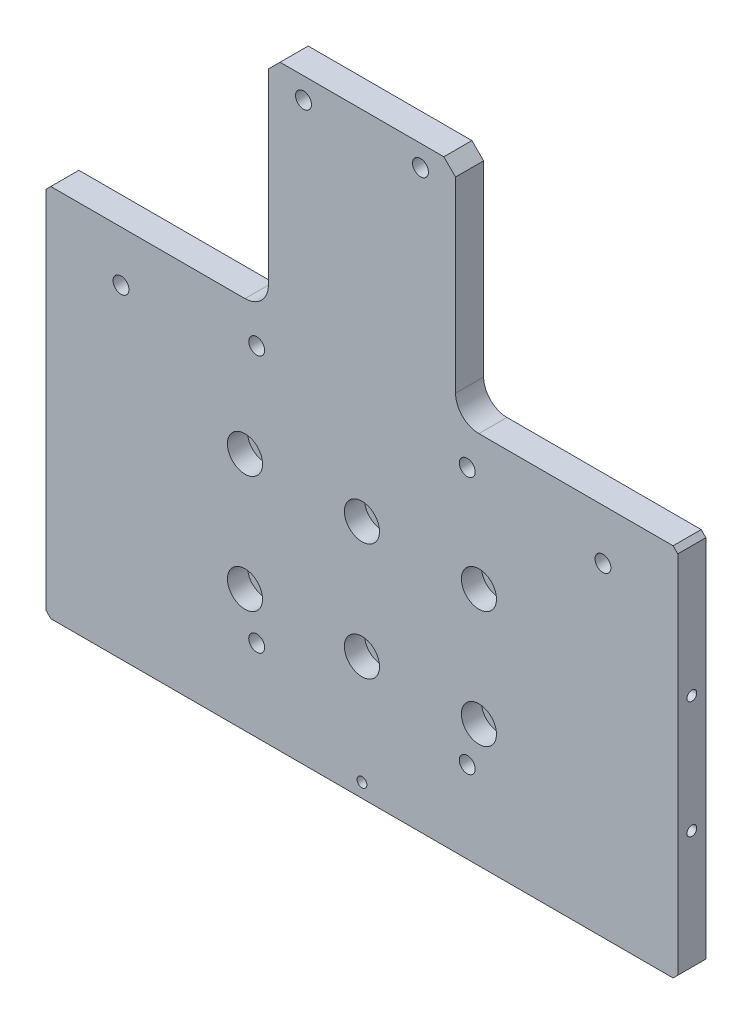
from build123d import *

# Parameters (mm, degrees)
SKETCH_1_W                     = 270
SKETCH_1_H                     = 255
EXTRUDE_1_DEPTH                = 6
SKETCH_2_W                     = 95
SKETCH_2_H                     = 95
CUT_EXTRUDE_1_DEPTH            = 12
HOLE_WIZARD_M8_1_D             = 6.8
HOLE_WIZARD_M8_2_D             = 6.8
CHAMFER_1_SIZE                 = 5
CHAMFER_2_SIZE                 = 2
HOLE_WIZARD_M8_2_2_D           = 9
HOLE_WIZARD_M8_2_2_CBORE_D     = 15
HOLE_WIZARD_M8_2_2_CBORE_DEPTH = 8.6
FILLET_1_R                     = 10
HOLE_WIZARD_M5_3_AT_2_COUNT    = 2
HOLE_WIZARD_M5_3_AT_2_PITCH    = 50
HOLE_WIZARD_M5_4_D             = 4.2


with BuildPart() as part:
    # 草图1 → 凸台-拉伸1 (new, symmetric)
    with BuildSketch(Plane.XY):
        Rectangle(SKETCH_1_W, SKETCH_1_H)
    extrude(amount=EXTRUDE_1_DEPTH, both=True)

    # 草图2 → 切除-拉伸1 (cut)
    with BuildSketch(Plane(origin=(0, 0, -6), x_dir=(-1, 0, 0), z_dir=(0, 0, -1))):
        with Locations((87.5, 80)):
            Rectangle(SKETCH_2_W, SKETCH_2_H)
        with Locations((-87.5, 80)):
            Rectangle(SKETCH_2_W, SKETCH_2_H)
    extrude(amount=-CUT_EXTRUDE_1_DEPTH, mode=Mode.SUBTRACT)

    # Hole Wizard M8 _1 (through all)
    with Locations(Plane(origin=(0, 0, -6), x_dir=(-1, 0, 0), z_dir=(0, 0, -1))):
        with Locations((-25, 118.5), (25, 118.5)):
            Hole(HOLE_WIZARD_M8_1_D / 2)

    # Hole Wizard M8 _2 (through all)
    with Locations(Plane(origin=(0, 0, -6), x_dir=(-1, 0, 0), z_dir=(0, 0, -1))):
        with Locations((-45, -92.5), (45, -92.5), (-45, 17.5), (45, 17.5), (-103, 11), (103, 11)):
            Hole(HOLE_WIZARD_M8_2_D / 2)

    # 倒角1
    chamfer_1_edges = [part.edges().sort_by_distance(p)[0] for p in [
        (-40, 127.5, 0),
        (40, 127.5, 0),
    ]]
    chamfer(chamfer_1_edges, length=CHAMFER_1_SIZE)

    # 倒角2
    chamfer_2_edges = [part.edges().sort_by_distance(p)[0] for p in [
        (-135, 32.5, 0),
        (135, 32.5, 0),
        (135, -127.5, 0),
        (-135, -127.5, 0),
    ]]
    chamfer(chamfer_2_edges, length=CHAMFER_2_SIZE)

    # Hole Wizard M8 _2 2 (through all)
    with Locations(Plane.XY.offset(6)):
        with Locations((-50, -25), (-50, -75), (0, -25), (0, -75), (50, -25), (50, -75)):
            CounterBoreHole(HOLE_WIZARD_M8_2_2_D / 2, HOLE_WIZARD_M8_2_2_CBORE_D / 2, HOLE_WIZARD_M8_2_2_CBORE_DEPTH)

    # 圆角1
    fillet_1_edges = [part.edges().sort_by_distance(p)[0] for p in [
        (-40, 32.5, 0),
        (40, 32.5, 0),
    ]]
    fillet(fillet_1_edges, radius=FILLET_1_R)

    # 草图24 → M5 螺纹孔3 (revolve, cut)
    with BuildSketch(Plane(origin=(-135, -75, 0), x_dir=(0, 0, 1), z_dir=(0, 1, 0))):
        Polygon((0, 0), (0, 13.6618073), (2.1, 12.4), (2.1, 0), align=None)
    hole_wizard_m5_3 = revolve(axis=Axis((-141.35, -75, 0), (1, 0, 0)), mode=Mode.SUBTRACT)

    # M5 螺纹孔3 at 2: M5 螺纹孔3 ×2
    with Locations(*[(0, i * HOLE_WIZARD_M5_3_AT_2_PITCH, 0) for i in range(1, HOLE_WIZARD_M5_3_AT_2_COUNT)]):
        add(hole_wizard_m5_3, mode=Mode.SUBTRACT)

    # 镜向1: M5 螺纹孔3 across plane
    add(hole_wizard_m5_3.mirror(Plane.ZY), mode=Mode.SUBTRACT)

    # 镜向1 copy 1 sketch → 镜向1 copy 1 (revolve, cut)
    with BuildSketch(Plane(origin=(135, -25, 0), x_dir=(0, 0, 1), z_dir=(0, 1, 0))):
        Polygon((0, 0), (0, -13.6618073), (2.1, -12.4), (2.1, 0), align=None)
    revolve(axis=Axis((141.35, -25, 0), (1, 0, 0)), mode=Mode.SUBTRACT)

    # M5 螺纹孔4 (through all)
    with Locations(Plane.XY.offset(6)):
        with Locations((0, -121.5)):
            Hole(HOLE_WIZARD_M5_4_D / 2)


solid = part.part
